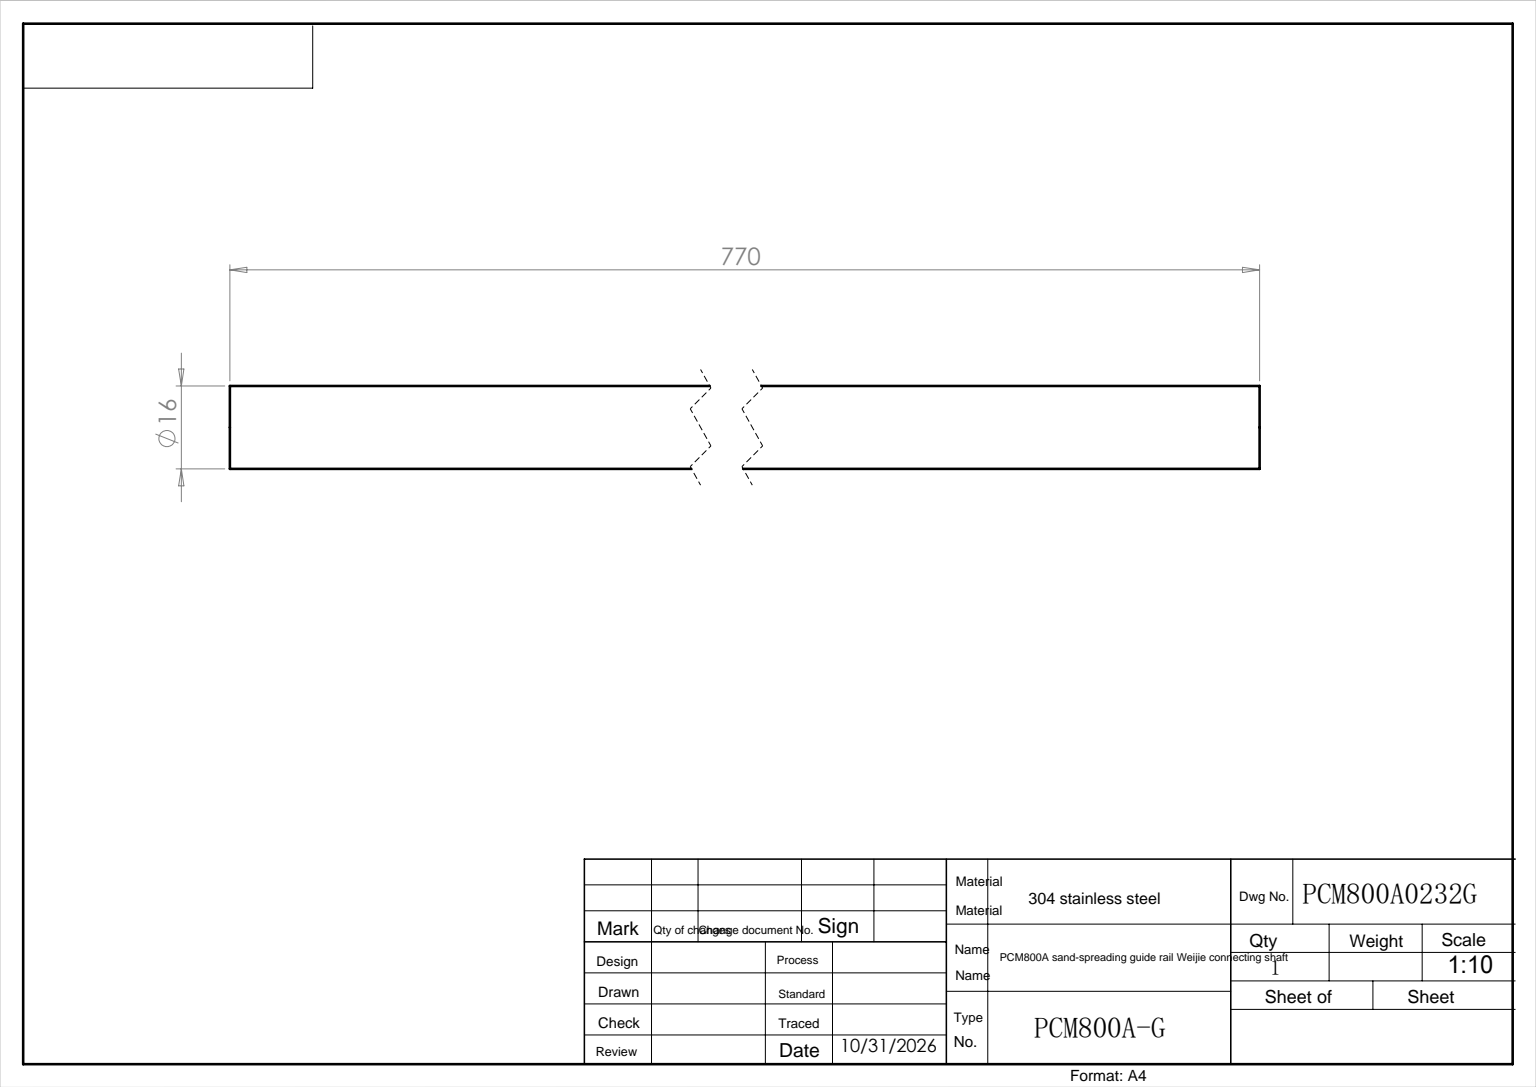
SolidWorks part; units mm, degrees
ref_plane "前视" through (0, 0, 0) normal (0, 0, 1) x (1, 0, 0)
ref_plane "上视" through (0, 0, 0) normal (0, 1, 0) x (1, 0, 0)
ref_plane "右视" through (0, 0, 0) normal (1, 0, 0) x (0, 0, -1)
sketch "草图1" plane through (0, 0, 0) normal (0, 0, 1) x (1, 0, 0)
  circle A0 centre (0, 0) radius 8
  dimension "D1" = 16
extrude "基体-拉伸" add sketch "草图1" along normal blind 770
